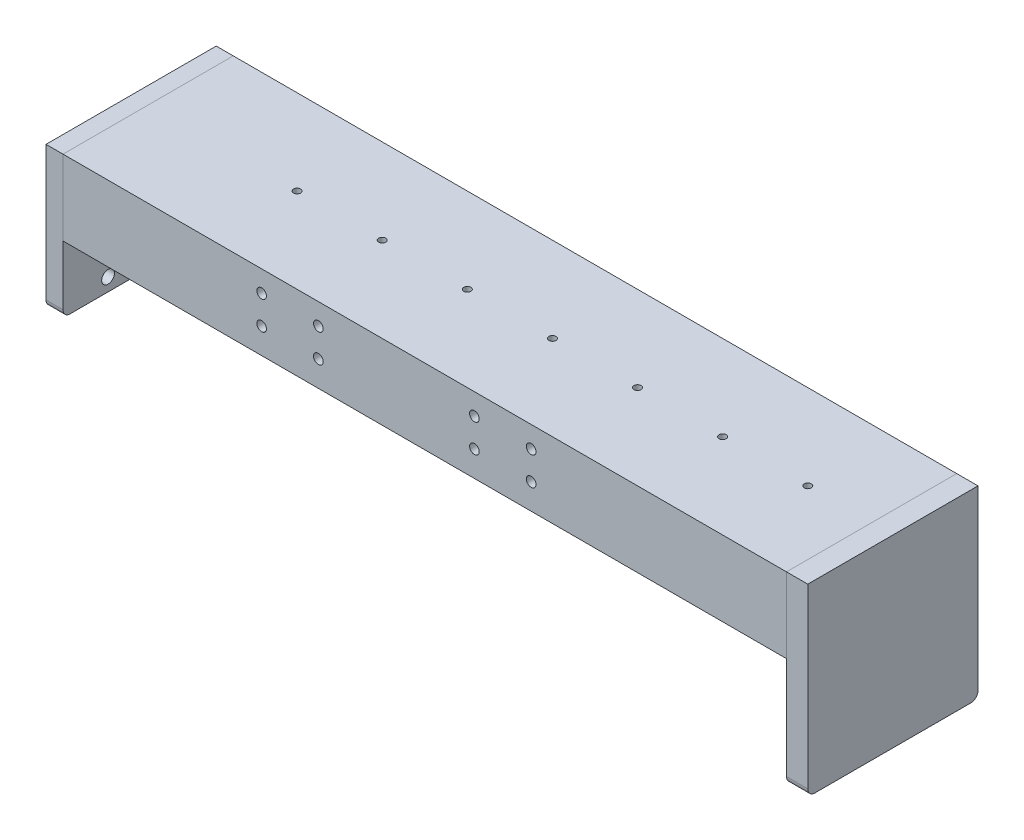
from build123d import *

# Parameters (mm, degrees)
MEMBER_1_DEPTH                   = 510
SKETCH_5_W                       = 120
SKETCH_5_H                       = 100
EXTRUDE_1_DEPTH                  = 12
SKETCH_6_W                       = 120
SKETCH_6_H                       = 130
EXTRUDE_2_DEPTH                  = 15
FILLET_1_R                       = 5
FILLET_2_R                       = 5
HOLE_WIZARD_M6_1_AT_2_COUNT      = 2
HOLE_WIZARD_M6_1_AT_2_PITCH      = 60
HOLE_WIZARD_M6_1_AT_3_COUNT      = 2
HOLE_WIZARD_M6_1_AT_3_PITCH      = 120
HOLE_WIZARD_M6_1_AT_4_COUNT      = 2
HOLE_WIZARD_M6_1_AT_4_PITCH      = 180
HOLE_WIZARD_M6_1_AT_5_COUNT      = 2
HOLE_WIZARD_M6_1_AT_5_PITCH      = 240
HOLE_WIZARD_M6_1_AT_6_COUNT      = 2
HOLE_WIZARD_M6_1_AT_6_PITCH      = 300
HOLE_WIZARD_M6_1_AT_7_COUNT      = 2
HOLE_WIZARD_M6_1_AT_7_PITCH      = 360
HOLE_WIZARD_M8_1_AT_2_COUNT      = 2
HOLE_WIZARD_M8_1_AT_2_PITCH      = 80
HOLE_WIZARD_M8_1_AT_3_COUNT      = 2
HOLE_WIZARD_M8_1_AT_3_PITCH      = 40
SKETCH_11_W                      = 3.4
SKETCH_11_H                      = 120
HOLE_WIZARD_M8_2_AT_2_COUNT      = 2
HOLE_WIZARD_M8_2_AT_2_PITCH      = 20
HOLE_WIZARD_M8_2_AT_3_COUNT      = 2
HOLE_WIZARD_M8_2_AT_3_PITCH      = 44.72135955
HOLE_WIZARD_M8_2_AT_4_COUNT      = 2
HOLE_WIZARD_M8_2_AT_4_PITCH      = 40
HOLE_WIZARD_9_0_9_1_AT_2_COUNT   = 2
HOLE_WIZARD_9_0_9_1_AT_2_PITCH   = 56.5
HOLE_WIZARD_9_0_9_1_AT_3_COUNT   = 2
HOLE_WIZARD_9_0_9_1_AT_3_PITCH   = 79.903066274
HOLE_WIZARD_9_0_9_1_AT_4_COUNT   = 2
HOLE_WIZARD_9_0_9_1_AT_4_PITCH   = 56.5
SKETCH_15_R                      = 25
CUT_EXTRUDE_1_DEPTH              = 20
PATTERN_LINEAR_1_COUNT           = 2
PATTERN_LINEAR_1_PITCH           = 150
PATTERN_LINEAR_1_COPY_1_SKETCH_W = 3.4
PATTERN_LINEAR_1_COPY_1_SKETCH_H = 120
PATTERN_LINEAR_1_COPY_2_SKETCH_W = 3.4
PATTERN_LINEAR_1_COPY_2_SKETCH_H = 120
PATTERN_LINEAR_1_COPY_3_SKETCH_W = 3.4
PATTERN_LINEAR_1_COPY_3_SKETCH_H = 120


with BuildPart() as part:
    # Sketch1 → Member 1 (new body)
    with BuildSketch(Plane.YZ):
        with BuildLine():
            Line((0, 0), (0, -120))
            Line((0, -120), (-53, -120))
            Line((-53, -120), (-53, -117.0157841))
            ThreePointArc((-53, -117.0157841), (-51.788791155, -113.944326346), (-48.807176562, -112.526280502))
            Line((-48.807176562, -112.526280502), (-13.885646876, -110.136912681))
            ThreePointArc((-13.885646876, -110.136912681), (-7.922417689, -107.300820993), (-5.5, -101.157905484))
            Line((-5.5, -101.157905484), (-5.5, -18.842094516))
            ThreePointArc((-5.5, -18.842094516), (-7.922417689, -12.699179007), (-13.885646876, -9.863087319))
            Line((-13.885646876, -9.863087319), (-48.807176562, -7.473719498))
            ThreePointArc((-48.807176562, -7.473719498), (-51.788791155, -6.055673654), (-53, -2.9842159))
            Line((-53, -2.9842159), (-53, 0))
            Line((-53, 0), (0, 0))
        make_face()
    extrude(amount=MEMBER_1_DEPTH)

    # 草图7 → M6 螺纹孔1 (revolve, cut)
    with BuildSketch(Plane(origin=(105, -5.5, -60), x_dir=(0, 0, -1), z_dir=(1, 0, 0))):
        Polygon((0, 0), (0, 16.502151548), (2.5, 15), (2.5, 0), align=None)
    hole_wizard_m6_1 = revolve(axis=Axis((105, -11.85, -60), (0, 1, 0)), mode=Mode.SUBTRACT)

    # M6 螺纹孔1 at 2: M6 螺纹孔1 ×2
    with Locations(*[(i * HOLE_WIZARD_M6_1_AT_2_PITCH, 0, 0) for i in range(1, HOLE_WIZARD_M6_1_AT_2_COUNT)]):
        add(hole_wizard_m6_1, mode=Mode.SUBTRACT)

    # M6 螺纹孔1 at 3: M6 螺纹孔1 ×2
    with Locations(*[(i * HOLE_WIZARD_M6_1_AT_3_PITCH, 0, 0) for i in range(1, HOLE_WIZARD_M6_1_AT_3_COUNT)]):
        add(hole_wizard_m6_1, mode=Mode.SUBTRACT)

    # M6 螺纹孔1 at 4: M6 螺纹孔1 ×2
    with Locations(*[(i * HOLE_WIZARD_M6_1_AT_4_PITCH, 0, 0) for i in range(1, HOLE_WIZARD_M6_1_AT_4_COUNT)]):
        add(hole_wizard_m6_1, mode=Mode.SUBTRACT)

    # M6 螺纹孔1 at 5: M6 螺纹孔1 ×2
    with Locations(*[(i * HOLE_WIZARD_M6_1_AT_5_PITCH, 0, 0) for i in range(1, HOLE_WIZARD_M6_1_AT_5_COUNT)]):
        add(hole_wizard_m6_1, mode=Mode.SUBTRACT)

    # M6 螺纹孔1 at 6: M6 螺纹孔1 ×2
    with Locations(*[(i * HOLE_WIZARD_M6_1_AT_6_PITCH, 0, 0) for i in range(1, HOLE_WIZARD_M6_1_AT_6_COUNT)]):
        add(hole_wizard_m6_1, mode=Mode.SUBTRACT)

    # M6 螺纹孔1 at 7: M6 螺纹孔1 ×2
    with Locations(*[(i * HOLE_WIZARD_M6_1_AT_7_PITCH, 0, 0) for i in range(1, HOLE_WIZARD_M6_1_AT_7_COUNT)]):
        add(hole_wizard_m6_1, mode=Mode.SUBTRACT)

    # 草图11 → M8 螺纹孔2 (revolve, cut)
    with BuildSketch(Plane(origin=(140, -15, -120), x_dir=(0, 1, 0), z_dir=(1, 0, 0))):
        with Locations((1.7, 60)):
            Rectangle(SKETCH_11_W, SKETCH_11_H)
    hole_wizard_m8_2 = revolve(axis=Axis((140, -15, -126.35), (0, 0, 1)), mode=Mode.SUBTRACT)

    # M8 螺纹孔2 at 2: M8 螺纹孔2 ×2
    with Locations(*[(0, -i * HOLE_WIZARD_M8_2_AT_2_PITCH, 0) for i in range(1, HOLE_WIZARD_M8_2_AT_2_COUNT)]):
        add(hole_wizard_m8_2, mode=Mode.SUBTRACT)

    # M8 螺纹孔2 at 3: M8 螺纹孔2 ×2
    with Locations(*[Vector(0.8944271909999159, -0.447213595499958, 0) * (i * HOLE_WIZARD_M8_2_AT_3_PITCH) for i in range(1, HOLE_WIZARD_M8_2_AT_3_COUNT)]):
        add(hole_wizard_m8_2, mode=Mode.SUBTRACT)

    # M8 螺纹孔2 at 4: M8 螺纹孔2 ×2
    with Locations(*[(i * HOLE_WIZARD_M8_2_AT_4_PITCH, 0, 0) for i in range(1, HOLE_WIZARD_M8_2_AT_4_COUNT)]):
        add(hole_wizard_m8_2, mode=Mode.SUBTRACT)

    # 阵列(线性)1: M8 螺纹孔2 ×2
    with Locations(*[(i * PATTERN_LINEAR_1_PITCH, 0, 0) for i in range(1, PATTERN_LINEAR_1_COUNT)]):
        add(hole_wizard_m8_2, mode=Mode.SUBTRACT)

    # 阵列(线性)1 copy 1 sketch → 阵列(线性)1 copy 1 (revolve, cut)
    with BuildSketch(Plane(origin=(290, -35, -120), x_dir=(0, 1, 0), z_dir=(1, 0, 0))):
        with Locations((1.7, 60)):
            Rectangle(PATTERN_LINEAR_1_COPY_1_SKETCH_W, PATTERN_LINEAR_1_COPY_1_SKETCH_H)
    revolve(axis=Axis((290, -35, -126.35), (0, 0, 1)), mode=Mode.SUBTRACT)

    # 阵列(线性)1 copy 2 sketch → 阵列(线性)1 copy 2 (revolve, cut)
    with BuildSketch(Plane(origin=(330, -35, -120), x_dir=(0, 1, 0), z_dir=(1, 0, 0))):
        with Locations((1.7, 60)):
            Rectangle(PATTERN_LINEAR_1_COPY_2_SKETCH_W, PATTERN_LINEAR_1_COPY_2_SKETCH_H)
    revolve(axis=Axis((330, -35, -126.35), (0, 0, 1)), mode=Mode.SUBTRACT)

    # 阵列(线性)1 copy 3 sketch → 阵列(线性)1 copy 3 (revolve, cut)
    with BuildSketch(Plane(origin=(330, -15, -120), x_dir=(0, 1, 0), z_dir=(1, 0, 0))):
        with Locations((1.7, 60)):
            Rectangle(PATTERN_LINEAR_1_COPY_3_SKETCH_W, PATTERN_LINEAR_1_COPY_3_SKETCH_H)
    revolve(axis=Axis((330, -15, -126.35), (0, 0, 1)), mode=Mode.SUBTRACT)


with BuildPart() as body_2:
    # 草图5 → 凸台-拉伸1 (new body)
    with BuildSketch(Plane.ZY):
        with Locations((-60, -50)):
            Rectangle(SKETCH_5_W, SKETCH_5_H)
    extrude(amount=EXTRUDE_1_DEPTH)

    # 圆角1
    fillet_1_edges = [body_2.edges().sort_by_distance(p)[0] for p in [
        (-6, -100, 0),
        (-6, -100, -120),
    ]]
    fillet(fillet_1_edges, radius=FILLET_1_R)

    # 草图13 → Ø9.0 (9) 直径孔1 (revolve, cut)
    with BuildSketch(Plane(origin=(0, -90.75, -31.75), x_dir=(0, 0, -1), z_dir=(0, 1, 0))):
        Polygon((0, 0), (0, 22.703872786), (4.5, 20), (4.5, 0), align=None)
    hole_wizard_9_0_9_1 = revolve(axis=Axis((6.35, -90.75, -31.75), (-1, 0, 0)), mode=Mode.SUBTRACT)

    # Ø9.0 (9) 直径孔1 at 2: Ø9.0 (9) 直径孔1 ×2
    with Locations(*[(0, i * HOLE_WIZARD_9_0_9_1_AT_2_PITCH, 0) for i in range(1, HOLE_WIZARD_9_0_9_1_AT_2_COUNT)]):
        add(hole_wizard_9_0_9_1, mode=Mode.SUBTRACT)

    # Ø9.0 (9) 直径孔1 at 3: Ø9.0 (9) 直径孔1 ×2
    with Locations(*[Vector(0, 0.7071067811865475, -0.7071067811865476) * (i * HOLE_WIZARD_9_0_9_1_AT_3_PITCH) for i in range(1, HOLE_WIZARD_9_0_9_1_AT_3_COUNT)]):
        add(hole_wizard_9_0_9_1, mode=Mode.SUBTRACT)

    # Ø9.0 (9) 直径孔1 at 4: Ø9.0 (9) 直径孔1 ×2
    with Locations(*[(0, 0, -i * HOLE_WIZARD_9_0_9_1_AT_4_PITCH) for i in range(1, HOLE_WIZARD_9_0_9_1_AT_4_COUNT)]):
        add(hole_wizard_9_0_9_1, mode=Mode.SUBTRACT)

    # 草图15 → 切除-拉伸1 (cut)
    with BuildSketch(Plane(origin=(0, 0, 0), x_dir=(0, 0, -1), z_dir=(1, 0, 0))):
        with Locations((60, -62.5)):
            Circle(SKETCH_15_R)
    extrude(amount=-CUT_EXTRUDE_1_DEPTH, mode=Mode.SUBTRACT)


with BuildPart() as body_3:
    # 草图6 → 凸台-拉伸2 (new body)
    with BuildSketch(Plane(origin=(510, 0, 0), x_dir=(0, 0, -1), z_dir=(1, 0, 0))):
        with Locations((60, -65)):
            Rectangle(SKETCH_6_W, SKETCH_6_H)
    extrude(amount=EXTRUDE_2_DEPTH)

    # 圆角2
    fillet_2_edges = [body_3.edges().sort_by_distance(p)[0] for p in [
        (517.5, -130, -120),
        (517.5, -130, 0),
    ]]
    fillet(fillet_2_edges, radius=FILLET_2_R)

    # 草图9 → M8 螺纹孔1 (revolve, cut)
    with BuildSketch(Plane(origin=(517.5, -130, -100), x_dir=(0, 0, -1), z_dir=(1, 0, 0))):
        Polygon((0, 0), (0, 21.792926105), (3.4, 19.75), (3.4, 0), align=None)
    hole_wizard_m8_1 = revolve(axis=Axis((517.5, -136.35, -100), (0, 1, 0)), mode=Mode.SUBTRACT)

    # M8 螺纹孔1 at 2: M8 螺纹孔1 ×2
    with Locations(*[(0, 0, i * HOLE_WIZARD_M8_1_AT_2_PITCH) for i in range(1, HOLE_WIZARD_M8_1_AT_2_COUNT)]):
        add(hole_wizard_m8_1, mode=Mode.SUBTRACT)

    # M8 螺纹孔1 at 3: M8 螺纹孔1 ×2
    with Locations(*[(0, 0, i * HOLE_WIZARD_M8_1_AT_3_PITCH) for i in range(1, HOLE_WIZARD_M8_1_AT_3_COUNT)]):
        add(hole_wizard_m8_1, mode=Mode.SUBTRACT)


solid = Compound([part.part, body_2.part, body_3.part])
